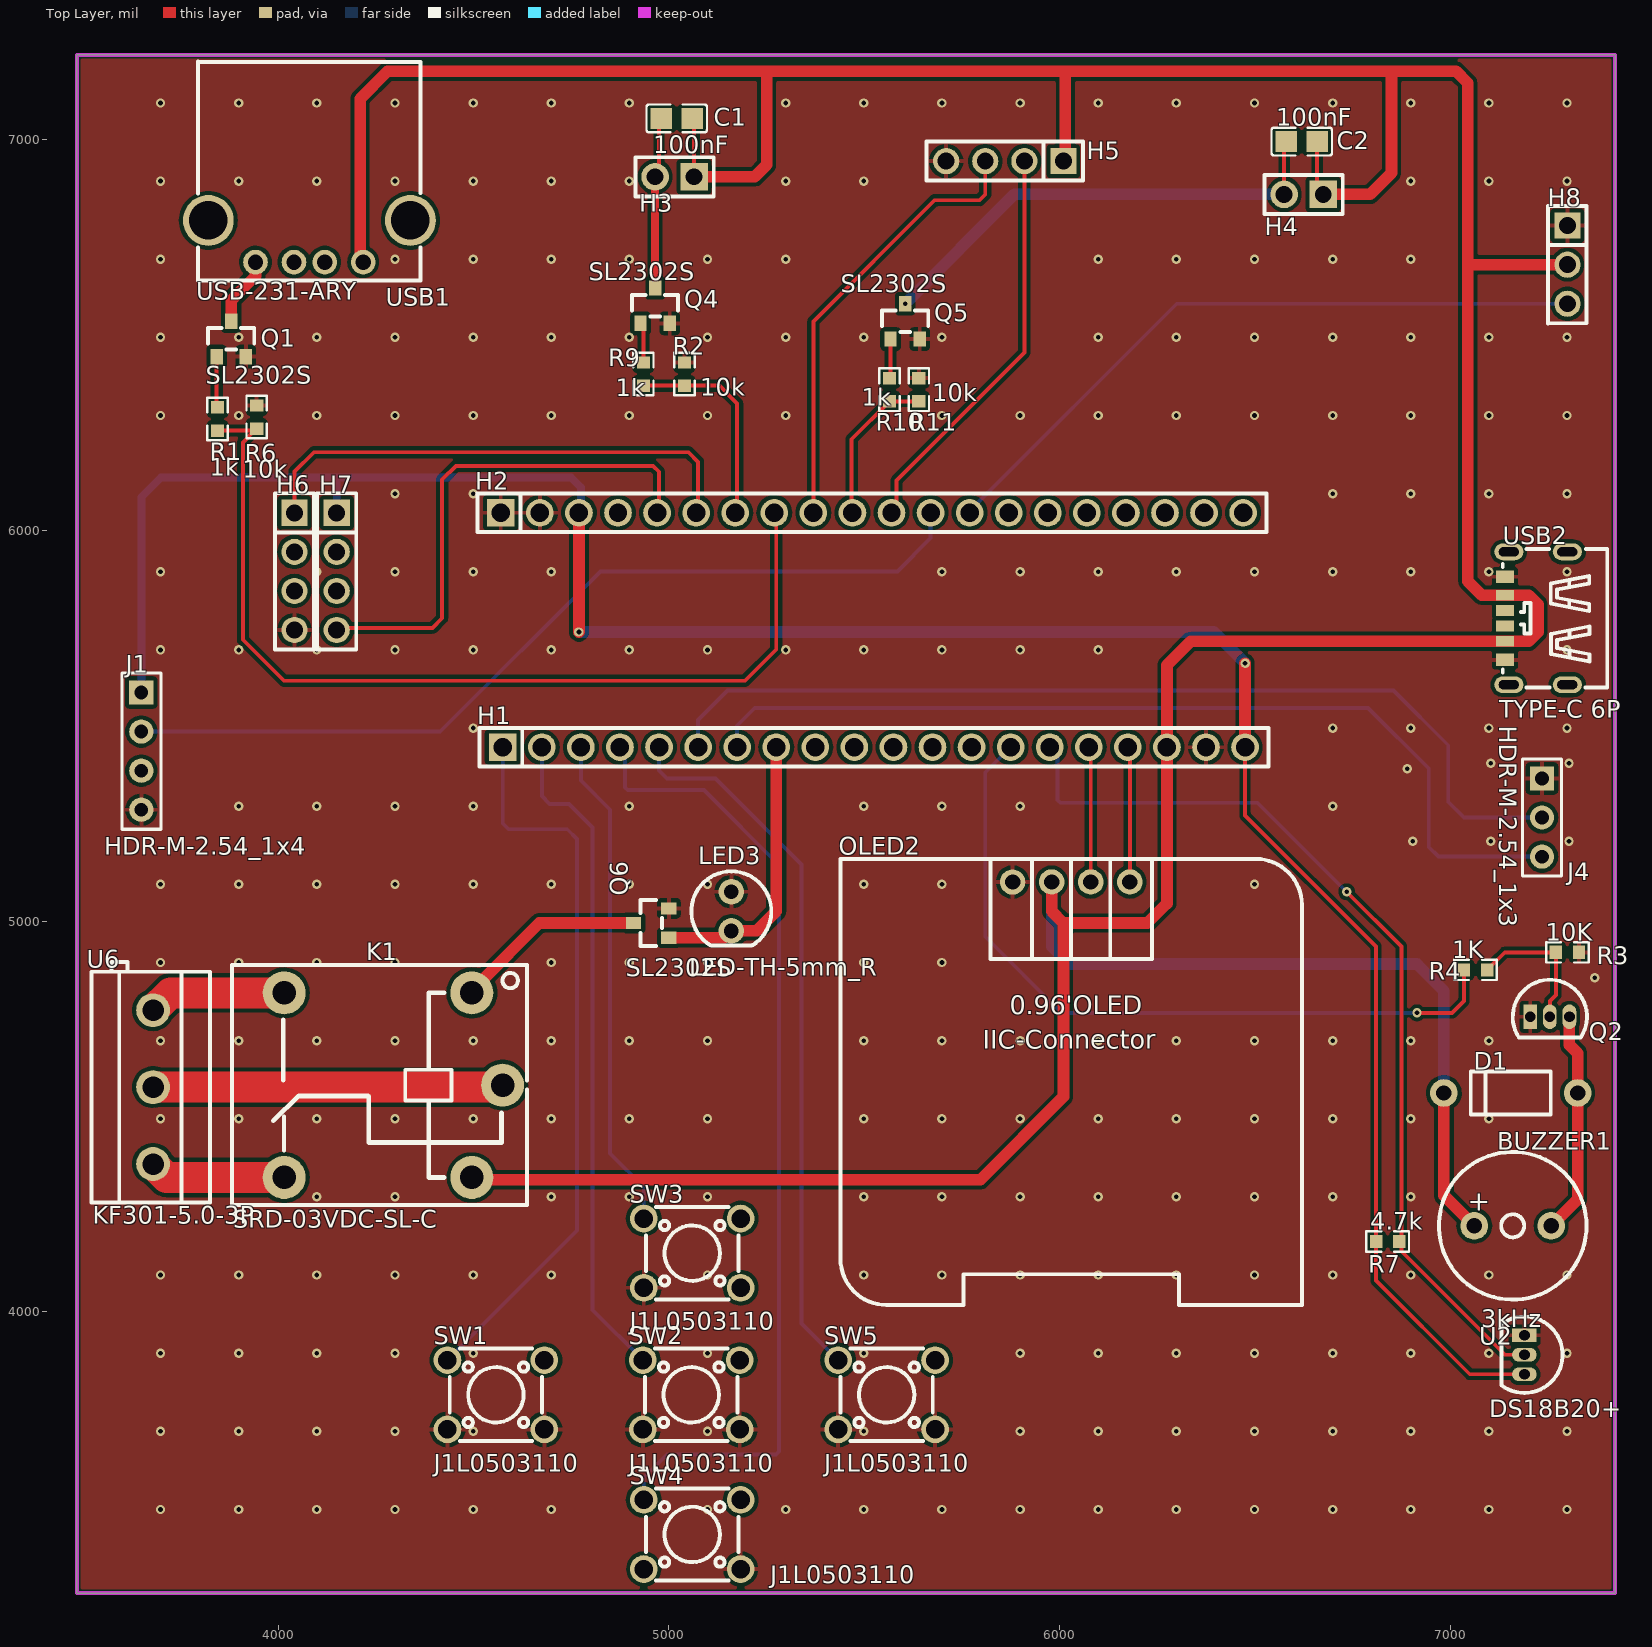
[diagram p0: Top Layer view]
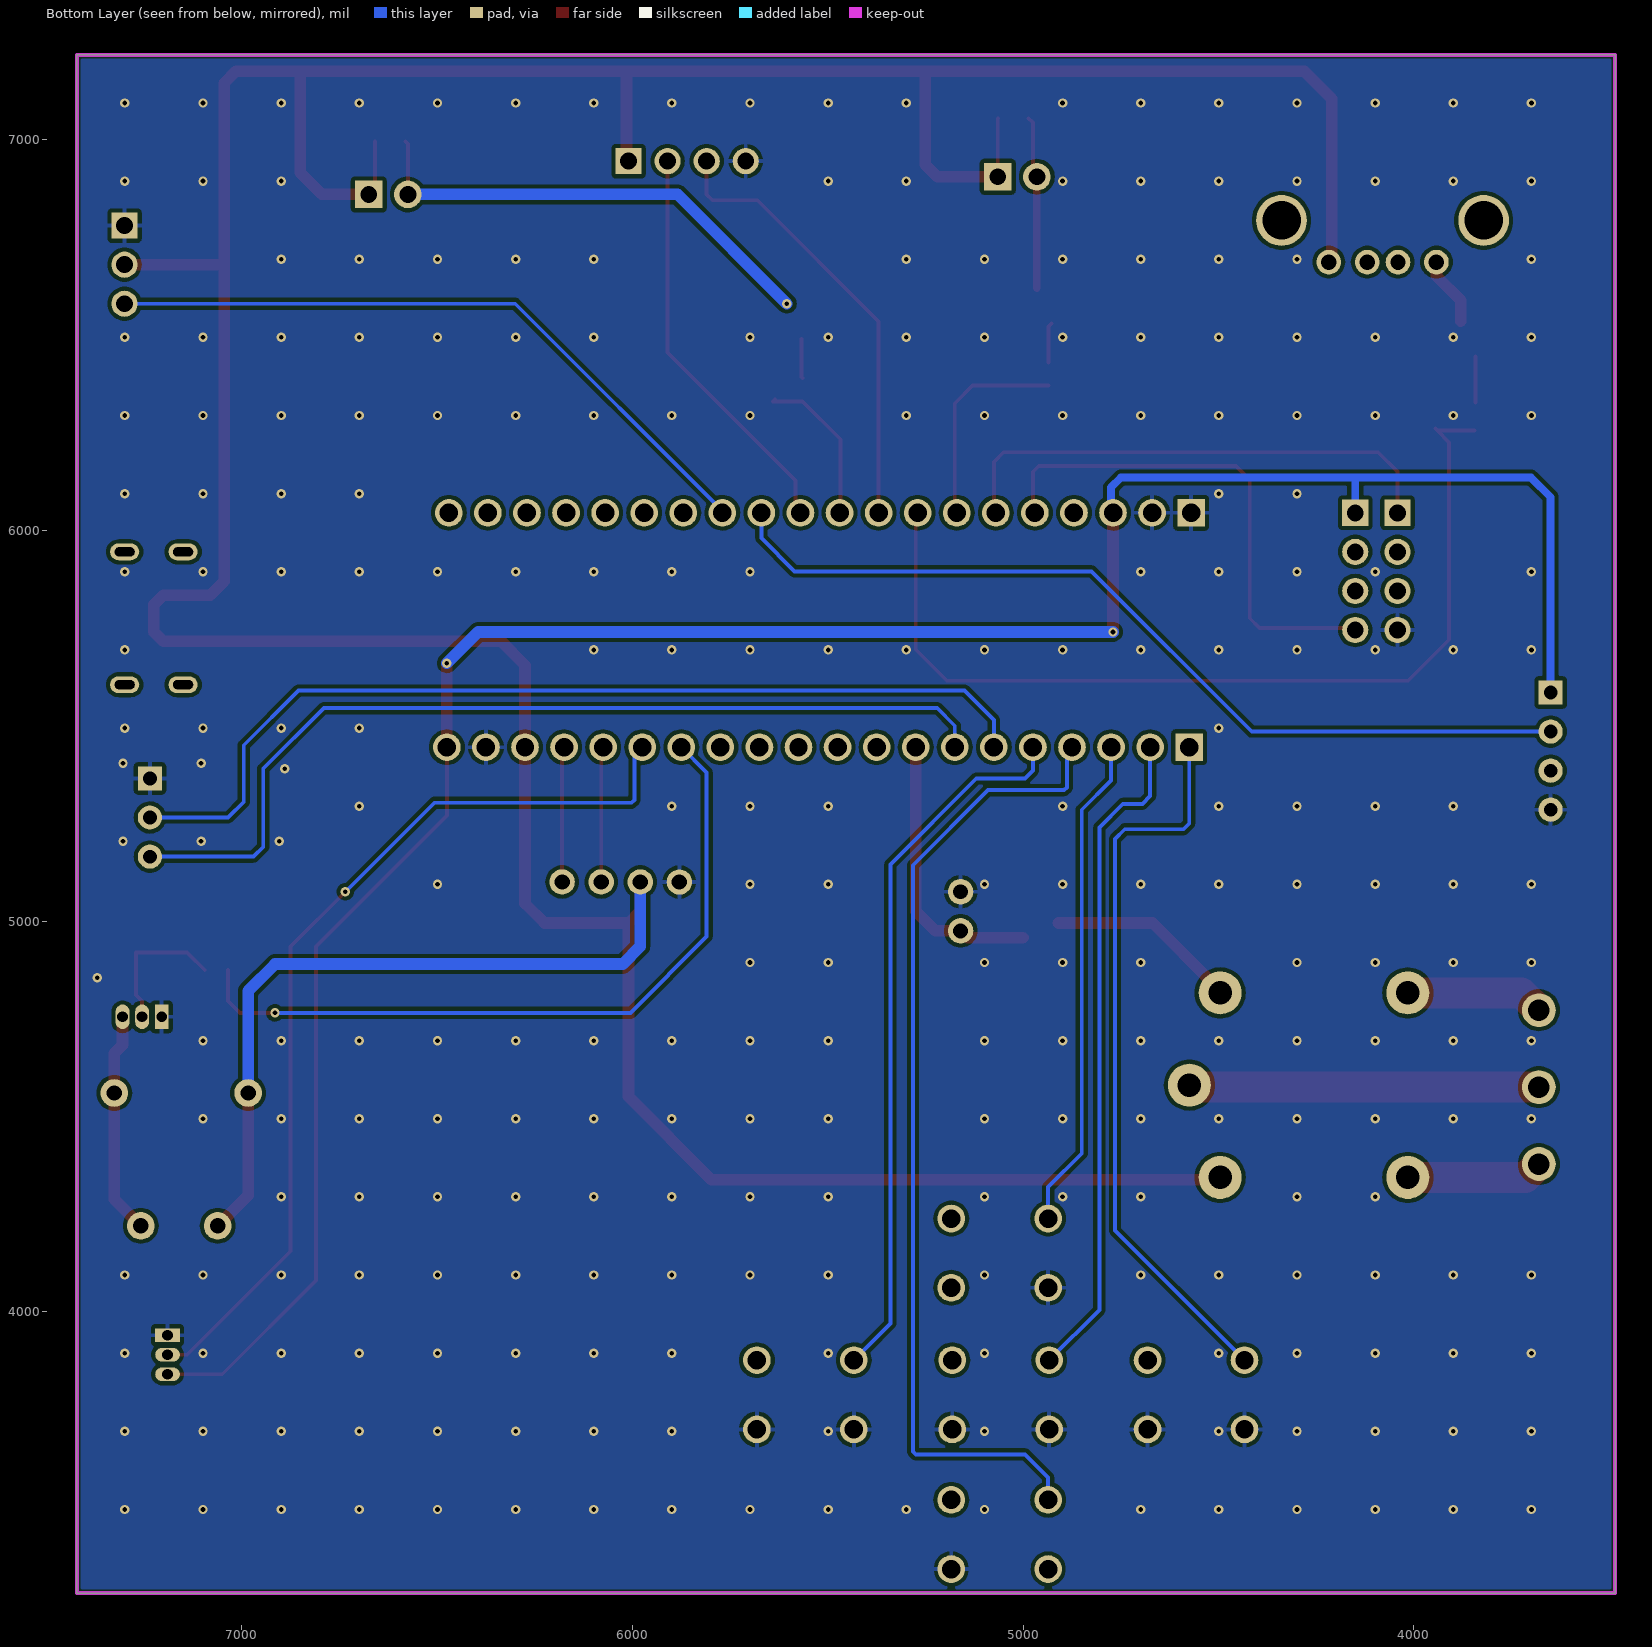
[diagram p1: Bottom Layer view, seen from below]
# Altium PCB MISC75353.pcbdoc
Units mil, origin at the board's own origin, x right, y up, seen from the top; angles counter-clockwise.
Board outline 3937 x 3937.11 mil, 2 copper layers (Top Layer, Bottom Layer), stack 62.206 mil thick; 40 components, 37 nets, 160 pads, 270 vias.

## Layer stack, top to bottom
Top Solder Mask Layer: solder mask 0.394, Dk 3.3
Top Layer: signal copper 1.379
Dielectric1: surface 59.449, FR4, Dk 4.5
Bottom Layer: signal copper 1.378
Bottom Solder Mask Layer: solder mask 0.394, Dk 3.3

## Board outline
3485,7217.01 3485,3279.9 7422,3279.9 7422,7217.01

## Design rules (kind name [scope] priority, off if disabled: settings)
BoardOutlineClearance copperThickness2oz_1 [All] p2 off: genericclearance=7.99 ignorepadtopadclearanceinfootprint=FALSE except(0: Arc-SplitContinuation Track-SplitContinuation SMDPad-SplitContinuation THPad-SplitContinuation Via-SplitContinuation Fill-SplitContinuation Region-SplitContinuation Poly-SplitContinuation Text-SplitContinuation Hole-SplitContinuation; 5.98: Arc-CutoutEdge SMDPad-CutoutEdge THPad-CutoutEdge Via-CutoutEdge Fill-CutoutEdge Region-CutoutEdge Text-CutoutEdge; 6.93: Hole-OutlineEdge Hole-CutoutEdge; 10: Poly-OutlineEdge Poly-CutoutEdge; 11.81: Arc-OutlineEdge Track-OutlineEdge SMDPad-OutlineEdge THPad-OutlineEdge Via-OutlineEdge Fill-OutlineEdge Region-OutlineEdge Text-OutlineEdge Track-CutoutEdge)
BoardOutlineClearance copperThickness1oz_1 [All] p4: genericclearance=4.02 ignorepadtopadclearanceinfootprint=FALSE except(0: Arc-SplitContinuation Track-SplitContinuation SMDPad-SplitContinuation THPad-SplitContinuation Via-SplitContinuation Fill-SplitContinuation Region-SplitContinuation Poly-SplitContinuation Text-SplitContinuation Hole-SplitContinuation; 6: SMDPad-CutoutEdge THPad-CutoutEdge Via-CutoutEdge Fill-CutoutEdge Region-CutoutEdge Text-CutoutEdge; 6.93: Hole-OutlineEdge Hole-CutoutEdge; 10: Poly-OutlineEdge Poly-CutoutEdge; 11.8: Arc-OutlineEdge Track-OutlineEdge SMDPad-OutlineEdge THPad-OutlineEdge Via-OutlineEdge Fill-OutlineEdge Region-OutlineEdge Text-OutlineEdge; 11.81: Arc-CutoutEdge Track-CutoutEdge)
Clearance copperThickness2oz [All] p1 off: gap=7.99 ignorepadtopadclearanceinfootprint=FALSE except(5.98: SMDPad-Track SMDPad-SMDPad THPad-Track SMDPad-THPad THPad-THPad Track-Via SMDPad-Via THPad-Via Via-Via Fill-Track Region-Track Fill-SMDPad Region-SMDPad Fill-THPad Region-THPad Fill-Via Region-Via Fill-Fill Fill-Region Region-Region Arc-Track Arc-SMDPad Arc-THPad Arc-Via Fill-Arc Region-Arc Arc-Arc Text-Track SMDPad-Text Text-THPad Text-Via Fill-Text Region-Text Arc-Text Text-Text; 6.93: Hole-Track Hole-SMDPad Hole-THPad Hole-Via Fill-Hole Region-Hole Hole-Arc Hole-Text; 10: Poly-Track Poly-SMDPad Poly-THPad Poly-Via Poly-Fill Poly-Region Poly-Poly Poly-Arc Poly-Text Poly-Hole)
Clearance copperThickness1oz [All] p3: gap=4.02 ignorepadtopadclearanceinfootprint=FALSE except(5.98: SMDPad-Track SMDPad-SMDPad THPad-Track SMDPad-THPad THPad-THPad Track-Via SMDPad-Via THPad-Via Via-Via Fill-Track Region-Track Fill-SMDPad Region-SMDPad Fill-THPad Region-THPad Fill-Via Region-Via Fill-Fill Fill-Region Region-Region; 6: Arc-Track Arc-SMDPad Arc-THPad Arc-Via Fill-Arc Region-Arc Arc-Arc Text-Track SMDPad-Text Text-THPad Text-Via Fill-Text Region-Text Arc-Text Text-Text; 6.93: Hole-Track Hole-SMDPad Hole-THPad Hole-Via Fill-Hole Region-Hole Hole-Arc Hole-Text; 10: Poly-Track Poly-SMDPad Poly-THPad Poly-Via Poly-Fill Poly-Region Poly-Poly Poly-Arc Poly-Text Poly-Hole)
DiffPairsRouting differentialPair [All] p1: maxlimit=6 minlimit=6 mostfreqgap=6 toplayer_minwidth=5 toplayer_prefwidth=10 toplayer_maxwidth=100 toplayer_mingap=6 toplayer_prefgap=6 toplayer_maxgap=6 bottomlayer_minwidth=5 bottomlayer_prefwidth=10 bottomlayer_maxwidth=100 bottomlayer_mingap=6 bottomlayer_prefgap=6 bottomlayer_maxgap=6 maxuncoupledlength=10
HoleToHoleClearance otherClearance [All] p1: gap=11.81 allowstackedmicrovias=TRUE
Length netLength [All] p1: minlimit=0 maxlimit=0
MatchedLengths netLengthTolerance [All] p1: tolerance=1000
PasteMaskExpansion pasteMaskExpansion [All] p1: expansion=0
PlaneConnect innerPlane [All] p1: planeconnectstyle=Relief reliefexpansion=20 reliefentries=4 reliefconductorwidth=10 reliefairgap=10
PolygonConnect copperRegion [(InNet('GND'))] p1: connectstyle=Relief reliefconductorwidth=10 reliefentries=4 polygonreliefangle="90 Angle" airgapwidth=10 via.connectstyle=Relief via.reliefconductorwidth=10 via.reliefentries=4 via.polygonreliefangle="90 Angle" via.airgapwidth=10
RoutingVias viaSize [All] p1: holewidth=12.01 width=24.02 viastyle="Through Hole" minholewidth=11.81 minwidth=19.68 maxholewidth=248.03 maxwidth=393.7
SolderMaskExpansion solderMaskExpansion [IsVia] p1: expansion=-1000 istentingtop=TRUE
SolderMaskExpansion solderMaskExpansion [All] p2: expansion=2 istentingtop=FALSE
Width copperThickness2oz_2 [All] p1 off: maxlimit=100 minlimit=8 preferedwidth=10
Width copperThickness1oz_2 [All] p2: maxlimit=100 minlimit=5 preferedwidth=10

## Components (designator, comment, footprint, x,y, rotation, side; value= is the part's Value field where it differs from the comment)
BUZZER1 "3kHz" BUZ-TH_BD9.6-P5.00-D0.7-FD 7160,4220 r0 top
C1 "100nF" C0805 5020.31,7054.47 r180 top
C2 "100nF" C0805 6620,6995 r180 top
D1 "" DO_1N4007 7155,4560 r0 top
H1 "" HDR-TH_20P-P2.54-V-F 5525,5445 r0 top
H2 "" HDR-TH_20P-P2.54-V-F 5520,6045 r0 top
H3 "" HDR-TH_2P-P2.54-V-M-1 5015,6905 r180 top
H4 "" HDR-TH_2P-P2.54-V-M-1 6625,6860 r180 top
H5 "" HDR-TH_4P-P2.54-V-M 5860,6945 r180 top
H6 "" HDR-TH_4P-P2.54-V-M 4041.84,5895 r270 top
H7 "" HDR-TH_4P-P2.54-V-M 4150,5895 r270 top
H8 "" HDR-TH_3P-P2.54-V-M 7300,6680 r270 top
J1 "HDR-M-2.54_1x4" HDR-M-2.54_1X4 3650,5435 r270 top
J4 "HDR-M-2.54_1x3" HDR-M-2.54_1X3 7235,5265 r270 top
K1 "SRD-03VDC-SL-C" RELAY-TH_SRD-XXVDC-XL-C 4295,4580 r180 top
LED3 "LED-TH-5mm_R" LED-TH_BD5.0_RED 5160,5025 r0 top
OLED2 "" 0.96OLED_4P 6030,5100 r0 top
Q1 "SL2302S" SOT-23_L2.9-W1.3-P1.90-LS2.4-BR 3880,6490 r270 top
Q2 "" S8050_TO_92 7255,4755 r0 top
Q4 "SL2302S" SOT-23_L2.9-W1.3-P1.90-LS2.4-BR 4965,6575 r270 top
Q5 "SL2302S" SOT-23_L2.9-W1.3-P1.90-LS2.4-BR 5605,6535 r270 top
Q6 "SL2302S" SOT-23_L2.9-W1.3-P1.90-LS2.4-BR 4955,4995 r0 top
R1 "1k" R0603 3845,6285 r90 top
R2 "10k" R0603 5040,6400 r90 top
R3 "10K" R0603 7300,4920 r180 top
R4 "1K" R0603 7065,4875 r180 top
R6 "10k" R0603 3945,6290 r90 top
R7 "4.7k" R0603 6840,4180 r180 top
R9 "1k" R0603 4935,6400 r90 top
R10 "1k" R0603 5565,6360 r90 top
R11 "10k" R0603 5640,6360 r90 top
SW1 "J1L0503110" SW-TH_4P-L6.0-W6.0-P4.50-LS6.3 4557.5,3787.5 r0 top
SW2 "J1L0503110" SW-TH_4P-L6.0-W6.0-P4.50-LS6.3 5057.5,3787.5 r0 top
SW3 "J1L0503110" SW-TH_4P-L6.0-W6.0-P4.50-LS6.3 5060,4150 r0 top
SW4 "J1L0503110" SW-TH_4P-L6.0-W6.0-P4.50-LS6.3 5060,3430 r0 top
SW5 "J1L0503110" SW-TH_4P-L6.0-W6.0-P4.50-LS6.3 5557.5,3787.5 r0 top
U2 "DS18B20+" TO-92-3_L4.9-W3.7-P1.27-L 7190,3890 r270 top
U6 "KF301-5.0-3P" CONN-TH_3P-P5.00_KF301-5.0-3P 3680,4575 r90 top
USB1 "USB-231-ARY" USB-A-TH_USB-231-ARY 4080,6740 r180 top
USB2 "TYPE-C 6P" TYPE-C-SMD_TYPE-C-6P_1 7220,5775 r90 top

## Footprints (in the part's own frame and the unit in brackets; to place one, negate y for a bottom-side part, rotate by r counter-clockwise, add the part's x,y. Pads: shape width x height; smd on the part's side, far side on the other; paste and mask are expansions set on the pad)
0.96OLED_4P [mm]
  round 1.65 hole 1 copper offset 0,0: 1(-3.81,-0.001) 2(-1.27,0.002) 3(1.27,0.002) 4(3.81,0.002)
  silkscreen extent -15,-27.5 15,1.5
BUZ-TH_BD9.6-P5.00-D0.7-FD [mm]
  round 1.8 hole 1: 1(-2.5,0) 2(2.5,0)
  silkscreen extent -4.8,-4.8 4.8,4.8
C0805 [mm]
  rect 1.41x1.35 smd paste-100 mask+0.051: 1(-1,0) 2(1,0)
  silkscreen extent -1.96,-0.9 1.96,0.9
CONN-TH_3P-P5.00_KF301-5.0-3P [mm]
  round 2.2 hole 1.4 paste+0 mask+0.051: 1(-5,0) 2(0,0) 3(5,0)
  silkscreen extent -7.5,-3.7 8.13,4
DO_1N4007 [mm]
  round 1.8 hole 1 paste+0 mask+0.051: 1(-4.35,0) 2(4.35,0)
  silkscreen extent -2.6,-1.4 2.6,1.4
HDR-M-2.54_1X3 [mil]
  rect 62x62 hole 35 paste+0 mask+2: 1(-100,0)
  round 62 hole 35 paste+0 mask+2: 2(0,0) 3(100,0)
  silkscreen extent -150,-50 150,50
HDR-M-2.54_1X4 [mil]
  rect 62x62 hole 35 paste+0 mask+2: 1(-150,0)
  round 62 hole 35 paste+0 mask+2: 2(-50,0) 3(50,0) 4(150,0)
  silkscreen extent -200,-50 200,50
HDR-TH_2P-P2.54-V-M-1 [mm]
  rect 1.8x1.8 hole 1.1: 1(-1.27,0)
  round 1.8 hole 1.1: 2(1.27,0)
  silkscreen extent -2.54,-1.27 2.54,1.27
HDR-TH_3P-P2.54-V-M [mm]
  rect 1.7x1.7 hole 1.1: 1(-2.54,0)
  round 1.7 hole 1.1: 2(0,0) 3(2.54,0)
  silkscreen extent -3.81,-1.25 3.81,1.25
HDR-TH_4P-P2.54-V-M [mm]
  rect 1.7x1.7 hole 1.1: 1(-3.81,0)
  round 1.7 hole 1.1: 2(-1.27,0) 3(1.27,0) 4(3.81,0)
  silkscreen extent -5.08,-1.27 5.08,1.27
HDR-TH_20P-P2.54-V-F [mm]
  rect 1.8x1.8 hole 1.2: 1(-24.13,0)
  round 1.8 hole 1.2: 2(-21.59,0) 3(-19.05,0) 4(-16.51,0) 5(-13.97,0) 6(-11.43,0) 7(-8.89,0) 8(-6.35,0) 9(-3.81,0) 10(-1.27,0) 11(1.27,0) 12(3.81,0) 13(6.35,0) 14(8.89,0) 15(11.43,0) 16(13.97,0) 17(16.51,0) 18(19.05,0) 19(21.59,0) 20(24.13,0)
  silkscreen extent -25.65,-1.25 25.65,1.25
LED-TH_BD5.0_RED [mil]
  round 65 hole 38 paste+0 mask+2: 1(0,50) 2(0,-50)
  silkscreen extent -102,-88 102,102
R0603 [mil]
  rect 31.75x34.02 smd paste-3937.01 mask+2: 1(-29.66,-0.01) 2(29.66,0.01)
  silkscreen extent -55,-26 55,26
RELAY-TH_SRD-XXVDC-XL-C [mil]
  round 110 hole 60 paste+0 mask+2: 1(-200.79,-236.22) 2(279.53,-236.2) 3(279.53,236.2) 4(-200.79,236.22) 5(-279.53,0)
  silkscreen extent -342,-307 413,307
S8050_TO_92 [mil]
  rect 35.4x63 hole 27.6 paste+0 mask+2: 1(-50,0)
  oval 35.4x63 hole 27.6 paste+0 mask+2: 2(0,0) 3(50,0)
  silkscreen extent -95,-53 95,95
SOT-23_L2.9-W1.3-P1.90-LS2.4-BR [mm]
  rect 1x0.8 smd paste+0 mask+0.051: 1(1.15,-0.95) 2(1.15,0.95) 3(-1.15,0)
  silkscreen extent -0.7,-1.5 0.7,1.5
SW-TH_4P-L6.0-W6.0-P4.50-LS6.3 [mm]
  round 1.8 hole 1.2: 1(-3.15,2.25) 2(3.15,2.25) 3(-3.15,-2.25) 4(3.15,-2.25)
  silkscreen extent -3,-3 3,3
TO-92-3_L4.9-W3.7-P1.27-L [mm]
  rect 0.9x1.6 hole 0.7 paste+0 mask+0.051: 1(-1.27,0)
  oval 0.9x1.6 hole 0.7 paste+0 mask+0.051: 2(0,0) 3(1.27,0)
  silkscreen extent -2.48,-1.5 2.48,2.48
TYPE-C-SMD_TYPE-C-6P_1 [mm]
  oval 1.1x1.9 hole 0.6 slot 1.3 at 90 deg paste+0 mask+0.051: 7(-4.32,1.775) 7(-4.32,-2.025) 7(4.32,1.775)
  oval 1.1x1.9 hole 0.6 slot 1.3 at 90 deg copper offset 0,0 paste+0 mask+0.051: 7(4.32,-2.025)
  rect 0.7x1.2 smd paste-100 mask+0.051: A5(-0.5,2.025) A9(1.5,2.025) B5(0.5,2.025) B9(-1.5,2.025)
  rect 0.8x1.2 smd paste-100 mask+0.051: A12(2.7,2.025) B12(-2.7,2.025)
  silkscreen extent -4.5,-4.63 4.5,2.18
USB-A-TH_USB-231-ARY [mm]
  round 1.6 hole 1: 1(-3.5,1.355) 2(-1,1.355) 3(1,1.355) 4(3.5,1.355)
  round 3.3 hole 2.5: 5(-6.57,-1.355) 6(6.57,-1.355)
  silkscreen extent -7.23,-11.68 7.24,2.54

## Via types
v1: diameter 24.02, hole 12, Top Layer to Bottom Layer, 270 vias

## Nets (pads, with @x,y where several pads share a name; then routed paths per layer and width w, separated by ;. In a path a pad name is that pad's centre, name@x,y a point inside that pad or via, vN(x,y) a via of type N, cw(c..) or ccw(c..) an arc to the next point about the centre after c; other vN are vias at no path point)
$1N2: Q1.3 USB1.4 | length 177.2
  Top Layer w30: Q1.3 3880,6588.86 3942.21,6651.07 USB1.4
$1N4: Q1.1 R1.2 | length 117
  Top Layer w10: R1.2@3842.6,6327.74 Q1.1
$1N10: BUZZER1.2 D1.2 Q2.3 | length 571.9
  Top Layer w30: BUZZER1.2 7326.26,4287.84 D1.2 7326.26,4661.65 7305,4682.91 Q2.3
$1N26: Q4.1 R9.2 | length 103.1
  Top Layer w10: Q4.1 4935,6522.32 R9.2
$1N27: C1.2 H3.2 Q4.3 | length 442.9
  Top Layer w10: H3.2 4975,6915 4975,7043.54 C1.2@4985.94,7054.47
  Top Layer w20: Q4.3 H3.2
$1N30: C2.2 H4.2 Q5.3 | length 1223.2
  Top Layer w10: H4.2 6575,6989.37 C2.2
  Bottom Layer w30: v1(5605,6580.27) 5884.73,6860 H4.2
$1N32: Q5.1 R10.2 | length 101.1
  Top Layer w10: R10.2 5567.6,6392.26 Q5.1
$1N35: K1.2 U6.3 | length 353.8
  Top Layer w80: U6.3 3724.35,4816.2 K1.2
$1N38: K1.5 U6.2 | length 896.6
  Top Layer w80: U6.2 4569.53,4575 K1.5
$1N39: K1.3 U6.1 | length 349.7
  Top Layer w80: U6.1 3714.35,4343.8 K1.3
$1N121: K1.1 Q6.3 | length 457.1
  Top Layer w30: K1.1@4515.89,4842.23 4668.66,4995 Q6.3
$1N124: Q2.2 R3.2 R4.1 | length 365.7
  Top Layer w10: R4.1 7139.66,4920 R3.2 7270.34,4810.34 7255,4795 Q2.2
+5V: BUZZER1.1 C1.1 C2.1 D1.1 H1.18 H3.1 H4.1 H5.1 H8.2 K1.4 OLED2.2 USB1.1 USB2.A9 USB2.B9 | length 12373.8
  Top Layer w10: C1.1@5064.68,7054.47 5065,7054.15 H3.1 ; C2.1 6659.37,6875.63 H4.1
  Top Layer w30: USB1.1 4210,6694.45 4210,7105 4280,7175 5250.56,7175 ; K1.4@4528.61,4337.87 5797.87,4337.87 6010,4550 6010,4995 ; H3.1 5220,6905 5250.56,6935.56 5250.56,7175 ; OLED2.2@5980,5100.05 5980,5025 6010,4995 ; H5.1@6015,6955 6015,7175 ; H4.1 6795,6860 6850,6915 6850,7173.29 6851.71,7175 ; D1.1 6983.74,4297.84 BUZZER1.1 ; H8.2 7049.06,6680 7045,6675.94 ; 5250.56,7175 6015,7175 ; 6010,4995 6225,4995 6275,5045 H1.18 6275,5655 6335.95,5715.95 7140.27,5715.95 7200.95,5715.95 7225,5740 7225,5810 7200.94,5834.06 USB2.A9 7080.94,5834.06 7045,5870 7045,6675.94 ; 6015,7175 6851.71,7175 ; 6851.71,7175 7015,7175 7045,7145 7045,6675.94
  Bottom Layer w30: OLED2.2@5980,5100.05 5980,4935 6025,4890 6915,4890 6983.74,4821.26 D1.1
GND: H1.19 H2.1 H2.2 H5.4 H6.4 H8.1 J1.4 J4.1 LED3.1 OLED2.1 Q1.2 Q2.1 Q4.2 Q5.2 Q6.2 R2.2 R3.1 R6.2 R11.2 SW1.3 SW1.4 SW2.3 SW2.4 SW3.3 SW4.4 SW5.3 SW5.4 U2.1 USB2.A12 USB2.B12
  other v1: 3699.1,3494 3899.1,3494 4099.1,3494 4299.1,3494 4499.1,3494 4699.1,3494 5099.1,3494 5299.1,3494 5499.1,3494 5699.1,3494 5899.1,3494 6099.1,3494 6299.1,3494 6499.1,3494 6699.1,3494 6899.1,3494 7099.1,3494 7299.1,3494 3699.1,3694 3899.1,3694 4099.1,3694 4299.1,3694 4499.1,3694 5099.1,3694 5499.1,3694 5899.1,3694 6099.1,3694 6299.1,3694 6499.1,3694 6699.1,3694 6899.1,3694 7099.1,3694 7299.1,3694 3699.1,3894 3899.1,3894 4099.1,3894 4299.1,3894 4499.1,3894 5099.1,3894 5499.1,3894 5899.1,3894 6099.1,3894 6299.1,3894 6499.1,3894 6699.1,3894 6899.1,3894 7099.1,3894 7299.1,3894 3699.1,4094 3899.1,4094 4099.1,4094 4299.1,4094 4499.1,4094 4699.1,4094 5099.1,4094 5499.1,4094 5699.1,4094 5899.1,4094 6099.1,4094 6299.1,4094 6499.1,4094 6699.1,4094 6899.1,4094 7099.1,4094 7299.1,4094 4099.1,4294 4299.1,4294 4699.1,4294 4899.1,4294 5099.1,4294 5499.1,4294 5699.1,4294 5899.1,4294 6099.1,4294 6299.1,4294 6499.1,4294 6699.1,4294 6899.1,4294 3699.1,4494 3899.1,4494 4099.1,4494 4299.1,4494 4499.1,4494 4699.1,4494 4899.1,4494 5099.1,4494 5499.1,4494 5699.1,4494 5899.1,4494 6099.1,4494 6299.1,4494 6499.1,4494 6699.1,4494 6899.1,4494 7099.1,4494 3699.1,4694 3899.1,4694 4099.1,4694 4299.1,4694 4499.1,4694 4699.1,4694 4899.1,4694 5099.1,4694 5499.1,4694 5699.1,4694 5899.1,4694 6099.1,4694 6299.1,4694 6499.1,4694 6699.1,4694 6899.1,4694 7099.1,4694 7370,4855 3699.1,4894 3899.1,4894 4099.1,4894 4299.1,4894 4699.1,4894 4899.1,4894 5099.1,4894 5499.1,4894 5699.1,4894 3699.1,5094 3899.1,5094 4099.1,5094 4299.1,5094 4499.1,5094 4699.1,5094 4899.1,5094 5099.1,5094 5499.1,5094 5699.1,5094 6499.1,5094 6904.1,5204 7104.1,5204 7304.1,5204 3899.1,5294 4099.1,5294 4299.1,5294 4499.1,5294 4899.1,5294 5499.1,5294 5699.1,5294 5899.1,5294 6699.1,5294 6890,5390 7104.1,5404 7304.1,5404 4499.1,5494 6699.1,5494 6899.1,5494 7099.1,5494 7299.1,5494 3699.1,5694 3899.1,5694 4099.1,5694 4299.1,5694 4499.1,5694 4699.1,5694 4899.1,5694 5099.1,5694 5299.1,5694 5499.1,5694 5699.1,5694 5899.1,5694 6099.1,5694 7299.1,5694 3699.1,5894 4099.1,5894 4299.1,5894 4499.1,5894 4699.1,5894 5699.1,5894 5899.1,5894 6099.1,5894 6299.1,5894 6499.1,5894 6699.1,5894 6899.1,5894 7099.1,5894 7299.1,5894 4299.1,6094 4499.1,6094 6699.1,6094 6899.1,6094 7099.1,6094 7299.1,6094 3699.1,6294 3899.1,6294 4099.1,6294 4299.1,6294 4499.1,6294 4699.1,6294 4899.1,6294 5099.1,6294 5299.1,6294 5699.1,6294 5899.1,6294 6099.1,6294 6299.1,6294 6499.1,6294 6699.1,6294 6899.1,6294 7099.1,6294 7299.1,6294 3699.1,6494 3899.1,6494 4099.1,6494 4299.1,6494 4499.1,6494 4699.1,6494 4899.1,6494 5099.1,6494 5299.1,6494 5499.1,6494 5699.1,6494 6099.1,6494 6299.1,6494 6499.1,6494 6699.1,6494 6899.1,6494 7099.1,6494 7299.1,6494 3699.1,6694 4299.1,6694 4499.1,6694 4699.1,6694 4899.1,6694 5099.1,6694 5299.1,6694 6099.1,6694 6299.1,6694 6499.1,6694 6699.1,6694 6899.1,6694 3699.1,6894 3899.1,6894 4099.1,6894 4299.1,6894 4499.1,6894 4699.1,6894 4899.1,6894 5299.1,6894 5499.1,6894 6899.1,6894 7099.1,6894 7299.1,6894 3699.1,7094 3899.1,7094 4099.1,7094 4299.1,7094 4499.1,7094 4699.1,7094 4899.1,7094 5299.1,7094 5499.1,7094 5699.1,7094 5899.1,7094 6099.1,7094 6299.1,7094 6499.1,7094 6699.1,7094 6899.1,7094 7099.1,7094 7299.1,7094
PA3: H2.13 H8.3 | length 1754.5
  Bottom Layer w10: H2.13 5770,6050 6300,6580 H8.3
PA4: H2.12 J1.2 | length 2290
  Bottom Layer w10: J1.2 4415,5485 4825,5895 5585,5895 5670,5980 H2.12
PA5: H2.11 H5.2 | length 1040.8
  Top Layer w10: H2.11 5582.93,6057.93 5582.93,6127.93 5910,6455 H5.2
PA6: H2.10 R10.1 R11.1 | length 410.5
  Top Layer w10: H2.10@5475,6045 5467.93,6052.07 5467.93,6233.27 R10.1 R11.1@5630,6330.34 ; R11.1@5635,6335.34 R11.1@5630,6330.34 ; R11.1 R11.1@5630,6330.34
PA7: H2.9 H5.3 | length 1149.6
  Top Layer w10: H2.9 5370,6535 5680,6845 5795,6845 5810,6860 H5.3
PA8: H1.5 SW5.1 | length 1832.1
  Bottom Layer w10: H1.5 4975,5385 4995,5365 5120,5365 5340,5145 5340,3969.56 SW5.1
PA9: H1.6 J4.2 | length 2480.6
  Bottom Layer w10: H1.6 5075,5515 5150,5590 6855,5590 6995,5450 6995,5305 7035,5265 J4.2
PA10: H1.7 J4.3 | length 2408.2
  Bottom Layer w10: H1.7 5175,5500 5220,5545 6790,5545 6945,5390 6945,5190 6970,5165 J4.3
PA11: H1.8 LED3.2 Q6.1 | length 722.6
  Top Layer w30: Q6.1 5142.6,4957.6 LED3.2 5225,4975 5275,5025 H1.8
PB0: H2.8 R1.1 R6.1 | length 2441.5
  Top Layer w10: R1.1 R6.1@3940,6255.34 ; R6.1 R6.1@3940,6255.34 ; H2.8@5275,6045 5275,5695 5195,5615 4015,5615 3910,5720 3910,6225.34 R6.1@3940,6255.34
PB1: H2.7 R2.1 R9.1 | length 533.4
  Top Layer w10: R9.1 R2.1 5129.66,6370.34 5175,6325 H2.7@5175,6050.34
PB5: H1.13
PB6: H1.14 R4.2 | length 1910.3
  Top Layer w10: v1(6915,4765) 7005,4765 7035.34,4795.34 R4.2
  Bottom Layer w10: H1.14 5810,5380 5810,4960 6005,4765 v1(6915,4765)
PB7: H1.15 R7.1 U2.2 | length 2383.5
  Top Layer w10: v1(6735,5075) 6875,4935 6875,4154.8 7139.8,3890 U2.2
  Bottom Layer w10: H1.15 5995,5425 5995,5310 6002.07,5302.93 6507.07,5302.93 v1(6735,5075)
PB8: H1.16 OLED2.3 | length 347
  Top Layer w10: H1.16 6080,5440 OLED2.3@6080,5100.05
PB9: H1.17 OLED2.4 | length 347
  Top Layer w10: H1.17 6180,5440 OLED2.4@6180,5100.05
PB10: H2.6 H6.1 | length 1279.5
  Top Layer w10: H6.1@4041.84,6050 4041.84,6150.46 4091.38,6200 5050,6200 5075,6175 H2.6@5075,6060
PB11: H2.5 H7.4 | length 1316.1
  Top Layer w10: H7.4@4150,5750 4395,5750 4420,5775 4420,6130 4455,6165 4960,6165 4975,6150 H2.5@4975,6045
PB12: H1.1 SW1.1 | length 1872.8
  Bottom Layer w10: SW1.1 4765,4207.6 4765,5210 4740,5235 4590,5235 4575,5250 H1.1
PB13: H1.2 SW2.1 | length 1705.3
  Bottom Layer w10: H1.2 4675,5320 4695,5300 4745,5300 4805,5240 4805,4004.56 SW2.1
PB14: H1.3 SW3.1 | length 1273.1
  Bottom Layer w10: H1.3 4775,5360 4850,5285 4850,4405 4935.98,4319.02 SW3.1
PB15: H1.4 SW4.1 | length 2516.6
  Bottom Layer w10: H1.4 4887.93,5432.07 4887.93,5342.07 4895,5335 5090,5335 5282.07,5142.93 5282.07,3642.07 5275,3635 4995,3635 4935.98,3575.98 SW4.1
VCC: H1.20 H2.3 H7.1 J1.1 R7.2 U2.3 | length 6067.3
  Top Layer w10: H1.20 6475,5270 6810,4935 6810,4080 7050,3840 U2.3
  Top Layer w30: v1(4770,5740) H2.3 ; H1.20 v1(6475,5660)
  Bottom Layer w20: J1.1 3650,6085 3700,6135 4151.9,6135 ; H7.1 4150,6130 4151.9,6131.9 4151.9,6135 ; H2.3@4785,6035 4775,6045 4775,6110 4750,6135 4151.9,6135
  Bottom Layer w30: v1(4770,5740) 6395,5740 v1(6475,5660)
pads on no net: H1.9 H1.10 H1.11 H1.12 H2.4 H2.14 H2.15 H2.16 H2.17 H2.18 H2.19 H2.20 H6.2 H6.3 H7.2 H7.3 J1.3 SW1.2 SW2.2 SW3.2 SW3.4 SW4.2 SW4.3 SW5.2 USB1.2 USB1.3 USB1.5 USB1.6 USB2.7 USB2.A5 USB2.B5

## Polygon pours and split planes (outlines as drawn)
GND on Top Layer (solid, remove dead copper, pour order 0): 3000,7465 3000,3000 7905,3000 7905,7465
GND on Bottom Layer (solid, remove dead copper, pour order 2): 3315,7425 3315,3055 7620,3055 7620,7425

## Keep-outs
Board Outline Layer:
  the board outline again, w10